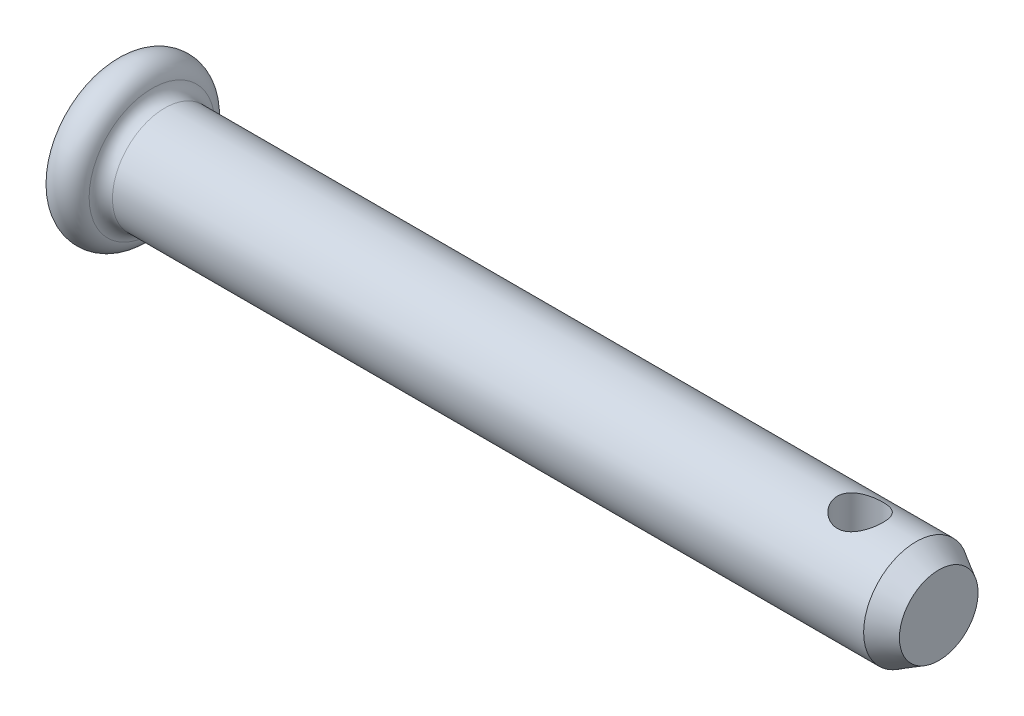
SolidWorks part; units mm, degrees
material "35钢"
ref_plane "前视" through (0, 0, 0) normal (0, 0, 1) x (1, 0, 0)
ref_plane "上视" through (0, 0, 0) normal (0, 1, 0) x (1, 0, 0)
ref_plane "右视" through (0, 0, 0) normal (1, 0, 0) x (0, 0, -1)
sketch "尺寸草图" plane through (0, 0, 0) normal (0, 0, 1) x (1, 0, 0)
  line L0 (0, 6) -> (0, 0)
  line L1 (0, 0) -> (30, 0)
  line L2 (30, 0) -> (33, 0) construction
  point P3 (0, 4)
  point P5 (1.5, 0)
  point P6 (0.5, 0)
  point P7 (29.5, 0)
  point P8 (3, 0)
  point P9 (0, 1.74)
sketch "草图1" plane through (0, 0, 0) normal (0, 0, 1) x (1, 0, 0)
  line L0 (0, 0) -> (10.7677, 0) construction
  line L1 (0, 0) -> (31.5, 0)
  line L2 (0, 0) -> (0, 2.25)
  line L4 (1.5, 2.25) -> (1.5, 2)
  line L5 (1.5, 2) -> (31.5, 2)
  line L6 (31.5, 2) -> (31.5, 0)
  arc A0 (0, 2.25) -> (1.5, 2.25) centre (0.75, 2.25) cw
revolve "基体-旋转" add sketch "草图1" angle 360 about L0
fillet "圆角1" radius 0.5 1 edges at (1.5, 0, 2)
chamfer "倒角1" distance 0.5 angle 60 1 edges at (31.5, 0, 2)
sketch "草图2" plane through (0, 0, 0) normal (0, 1, 0) x (1, 0, 0)
  circle A0 centre (28.5, 0) radius 0.87
extrude "切除-拉伸1" cut sketch "草图2" against normal mid plane 1000
equation "\"D4@草图1\" = \"K@尺寸草图\""
equation "\"D2@草图1\" = \"dk@尺寸草图\""
equation "\"D1@草图1\" = \"l@尺寸草图\""
equation "\"D3@草图1\" = \"d@尺寸草图\""
equation "\"D1@圆角1\" = \"r@尺寸草图\""
equation "\"D1@倒角1\" = \"c@尺寸草图\""
equation "\"D2@草图2\" = \"d1@尺寸草图\""
equation "\"lh@尺寸草图\" = \"l@尺寸草图\"-\"l-lh@尺寸草图\""
